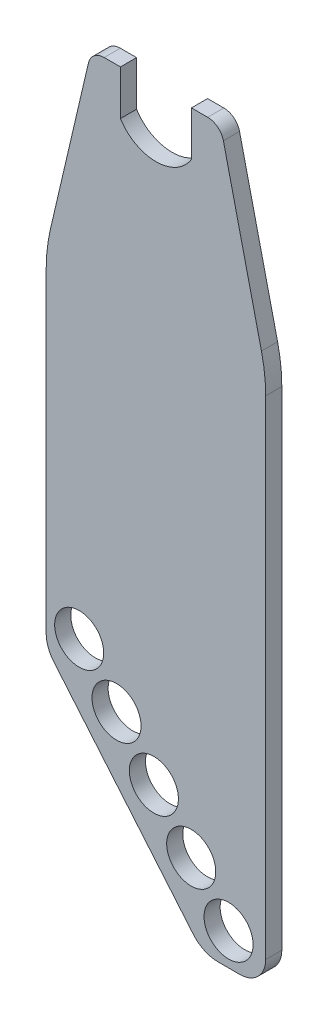
SolidWorks part; units mm, degrees
material "45#"
ref_plane "Front Plane" through (0, 0, 0) normal (0, 0, 1) x (1, 0, 0)
ref_plane "Top Plane" through (0, 0, 0) normal (0, 1, 0) x (1, 0, 0)
ref_plane "Right Plane" through (0, 0, 0) normal (1, 0, 0) x (0, 0, -1)
sketch "Sketch1" plane through (0, 0, 0) normal (0, 0, 1) x (1, 0, 0)
  line L1 (-34, 112.5) -> (34, 112.5)
  line L2 (-34, 112.5) -> (-34, -112.5)
  line L3 (-34, -112.5) -> (34, -112.5)
  line L4 (34, 112.5) -> (34, -112.5)
  line L5 (-34, 112.5) -> (34, -112.5) construction
  line L6 (-34, -112.5) -> (34, 112.5) construction
  point P0 (0, 0)
  dimension "D1" = 68
  dimension "D2" = 225
extrude "Boss-Extrude1" add sketch "Sketch1" along normal blind 5
sketch "Sketch3" plane through (0, 0, 5) normal (0, 0, 1) x (1, 0, 0)
  line L0 (34, -112.5) -> (34, 112.5) construction
  line L1 (-34, -112.5) -> (34, -112.5) construction
  line L2 (22.5, -102.5) -> (-43.0873, -24.336) construction
  circle A0 centre (22.5, -102.5) radius 7.6
  circle A1 centre (10.9298, -88.7112) radius 7.6
  circle A2 centre (-0.6404, -74.9224) radius 7.6
  circle A3 centre (-12.2105, -61.1336) radius 7.6
  circle A4 centre (-23.7807, -47.3448) radius 7.6
  dimension "D1" = 15.2
  dimension "D2" = 11.5
  dimension "D3" = 10
  dimension "D5" = 18
  dimension "D4" = 50
  dimension "D6" = 18
  dimension "D7" = 18
  dimension "D8" = 18
extrude "Cut-Extrude1" cut sketch "Sketch3" against normal blind 8
fillet "Fillet1" radius 8 1 edges at (34, -112.5, 2.5)
sketch "Sketch5" plane through (0, 0, 5) normal (0, 0, 1) x (1, 0, 0)
  line L0 (14.5734, -112.5) -> (-34, -54.6125)
  line L1 (-34, -112.5) -> (26, -112.5) construction
  line L2 (-34, -54.6125) -> (-34, -112.5)
  line L3 (-34, -112.5) -> (14.5734, -112.5)
  circle A1 centre (22.5, -102.5) radius 7.6 construction
  dimension "D1" = 50
  dimension "D2" = 12.5
extrude "Cut-Extrude2" cut sketch "Sketch5" against normal through all
fillet "Fillet2" radius 10 1 edges at (14.5734, -112.5, 2.5)
sketch "Sketch6" plane through (0, 0, 5) normal (0, 0, 1) x (1, 0, 0)
  line L1 (-11, 112.5) -> (-11, 98.6436)
  line L2 (34, 112.5) -> (-34, 112.5) construction
  line L3 (0, 112.5) -> (0, 105.5718) construction
  line L4 (11, 112.5) -> (11, 98.6436)
  arc A0 (-11, 98.6436) -> (11, 98.6436) centre (0, 105.5718) ccw
  arc A1 (11, 112.5) -> (-11, 112.5) centre (0, 105.5718) ccw
  dimension "D1" = 26
  dimension "D2" = 22
extrude "Cut-Extrude3" cut sketch "Sketch6" against normal blind 8
fillet "Fillet3" radius 10 1 edges at (-34, -54.6125, 2.5)
sketch "Sketch7" plane through (0, 0, 5) normal (0, 0, 1) x (1, 0, 0)
  line L0 (-20, 112.5) -> (-34, 52.5)
  line L1 (-11, 112.5) -> (-34, 112.5) construction
  line L2 (-34, 112.5) -> (-34, -50.9728) construction
  line L3 (-34, 52.5) -> (-34, 112.5)
  line L4 (-34, 112.5) -> (-20, 112.5)
  line L5 (0, 105.5718) -> (0, 47.5033) construction
  line L6 (34, 112.5) -> (20, 112.5)
  line L7 (34, 52.5) -> (34, 112.5)
  line L8 (20, 112.5) -> (34, 52.5)
  dimension "D1" = 40
  dimension "D2" = 60
extrude "Cut-Extrude4" cut sketch "Sketch7" against normal through all
fillet "Fillet4" radius 5 2 edges at (20, 112.5, 2.5) (-20, 112.5, 2.5)
fillet "Fillet5" radius 50 2 edges at (34, 52.5, 2.5) (-34, 52.5, 2.5)
